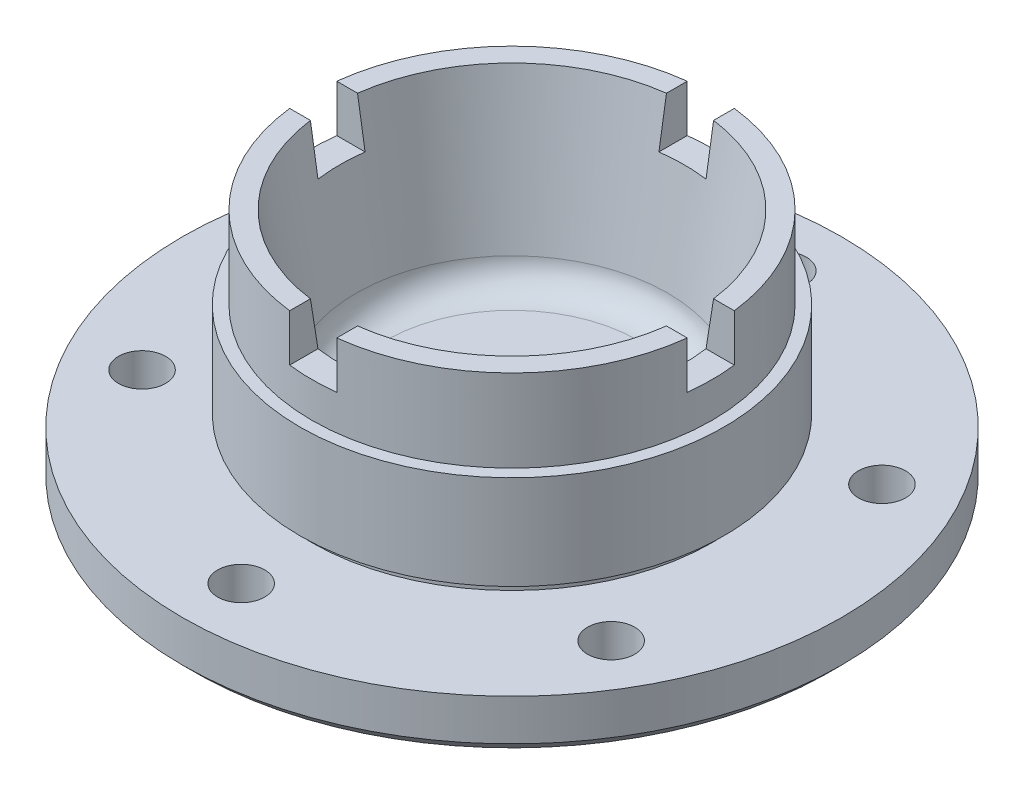
SolidWorks part; units mm, degrees
ref_plane "Front" through (0, 0, 0) normal (0, 0, 1) x (1, 0, 0)
ref_plane "Top" through (0, 0, 0) normal (0, 1, 0) x (1, 0, 0)
ref_plane "Right" through (0, 0, 0) normal (1, 0, 0) x (0, 0, -1)
sketch "Sketch1" plane through (0, 0, 0) normal (0, 0, 1) x (1, 0, 0)
  line L0 (0, 2) -> (0, 11)
  line L1 (0, 11) -> (0, 2)
  line L2 (0, 2) -> (31, 2)
  line L3 (31, 2) -> (32, 0)
  line L4 (54, 0) -> (56, 2)
  line L5 (32, 0) -> (54, 0)
  line L6 (56, 2) -> (56, 9)
  line L7 (56, 9) -> (34, 9)
  line L8 (34, 9) -> (34, 11)
  line L9 (34, 11) -> (36, 11)
  line L10 (36, 11) -> (36, 27)
  line L11 (36, 27) -> (34, 27)
  line L12 (34, 27) -> (34, 41)
  line L13 (0, 11) -> (16.5706, 11)
  line L14 (21.4751, 11) -> (16.5706, 11)
  line L15 (34, 41) -> (30.5, 41)
  line L18 (26.4502, 15.5025) -> (30.5, 41)
  arc A0 (26.4502, 15.5025) -> (21.4751, 11) centre (21.4751, 16) cw
  point P8 (56, 0)
  point P21 (26, 11)
  dimension "D15" = 5
  dimension "D3" = 31
  dimension "D5" = 9
  dimension "D6" = 22
  dimension "D7" = 2
  dimension "D8" = 2
  dimension "D9" = 16
  dimension "D10" = 2
  dimension "D11" = 14
revolve "Revolve1" add sketch "Sketch1" angle 360 about L0
sketch "Sketch2" plane through (0, 41, 0) normal (0, 1, 0) x (1, 0, 0)
  line L0 (48.2155, 4) -> (14.6829, 4)
  line L1 (-4, 48.2155) -> (4, 48.2155)
  line L2 (-4, 48.2155) -> (-4, 14.6829)
  line L3 (-4, 14.6829) -> (4, 14.6829)
  line L4 (4, 48.2155) -> (4, 14.6829)
  line L5 (48.2155, 4) -> (48.2155, -4)
  line L6 (48.2155, -4) -> (14.6829, -4)
  line L7 (14.6829, 4) -> (14.6829, -4)
  line L8 (4, -48.2155) -> (4, -14.6829)
  line L9 (4, -48.2155) -> (-4, -48.2155)
  line L10 (-4, -48.2155) -> (-4, -14.6829)
  line L11 (4, -14.6829) -> (-4, -14.6829)
  line L12 (-48.2155, -4) -> (-14.6829, -4)
  line L13 (-48.2155, -4) -> (-48.2155, 4)
  line L14 (-48.2155, 4) -> (-14.6829, 4)
  line L15 (-14.6829, -4) -> (-14.6829, 4)
  point P20 (0, 0)
  dimension "D1" = 8
  dimension "D2" = 4
  dimension "D3" = 4
extrude "Cut-Extrude1" cut sketch "Sketch2" against normal blind 8
sketch "Sketch3" plane through (0, 41, 0) normal (0, 1, 0) x (1, 0, 0)
  line L0 (0, 0) -> (66.5288, 0) construction
  line L1 (0, 0) -> (0, 55.2122) construction
  line L2 (0, 0) -> (56.892, 32.8466) construction
  line L3 (0, 0) -> (-57.5775, 33.2424) construction
  circle A0 centre (-39.8372, -23) radius 4
  circle A1 centre (0, 46) radius 4
  circle A2 centre (39.8372, 23) radius 4
  circle A3 centre (-39.8372, 23) radius 4
  circle A4 centre (0, -46) radius 4
  circle A5 centre (39.8372, -23) radius 4
  dimension "D4" = 8
  dimension "D5" = 8
  dimension "D1" = 60
  dimension "D2" = 60
extrude "Cut-Extrude2" cut sketch "Sketch3" against normal blind 94
scale "Scale 1" bodies to scale 103 scale about centroid uniform scaling yes scale factor 1.875
